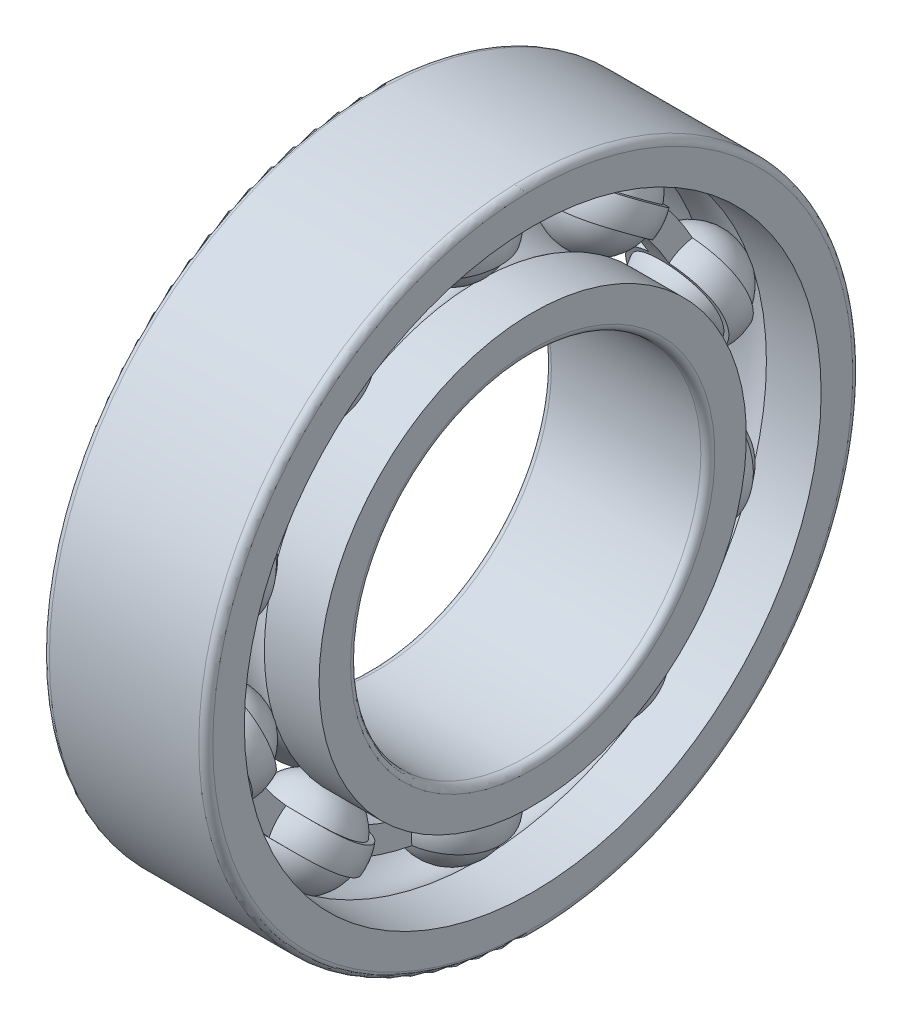
from build123d import *

# Parameters (mm, degrees)
SKETCH_2_W               = 0.87318
SKETCH_2_H               = 1.091475
PATTERN_CIRCULAR_1_COUNT = 10
SKETCH_4_W               = 4.3659
SKETCH_4_H               = 2.18295
SKETCH_5_W               = 4.3659
SKETCH_5_H               = 2.18295
PATTERN_CIRCULAR_2_COUNT = 10


with BuildPart() as part:
    # 草图2 → Revolve 262 (revolve)
    with BuildSketch(Plane.XY, mode=Mode.PRIVATE) as revolve_262_sk:
        with Locations((0, 10.75)):
            Rectangle(SKETCH_2_W, SKETCH_2_H)
    revolve(revolve_262_sk.sketch.rotate(Axis((-12.420610377, 0, 0), (1, 0, 0)), 90), axis=Axis((-12.420610377, 0, 0), (1, 0, 0)))

    # 草图3 → 凸台-旋转1 (revolve)
    with BuildSketch(Plane.XY):
        with BuildLine():
            Line((-2.18295, 10.75), (2.18295, 10.75))
            ThreePointArc((2.18295, 10.75), (0, 8.56705), (-2.18295, 10.75))
        make_face()
    revolve_1 = revolve(axis=Axis((-5.568093779, 10.75, 0), (1, 0, 0)))

    # 阵列(圆周)1: 凸台-旋转1 ×10 about axis
    pattern_circular_1_axis = Axis((0, 0, 0), (1, 0, 0))
    for i in range(1, PATTERN_CIRCULAR_1_COUNT):
        add(revolve_1.rotate(pattern_circular_1_axis, i * 360 / PATTERN_CIRCULAR_1_COUNT))

    # 草图4 → 切除-旋转1 (revolve, cut)
    with BuildSketch(Plane.XY, mode=Mode.PRIVATE) as cut_revolve_1_sk:
        with Locations((0, 12.3872125)):
            Rectangle(SKETCH_4_W, SKETCH_4_H)
    revolve(cut_revolve_1_sk.sketch.rotate(Axis((0, 0, 0), (1, 0, 0)), 82.768656666), axis=Axis((0, 0, 0), (1, 0, 0)), mode=Mode.SUBTRACT)

    # 草图5 → 切除-旋转2 (revolve, cut)
    with BuildSketch(Plane.XY, mode=Mode.PRIVATE) as cut_revolve_2_sk:
        with Locations((0, 9.1127875)):
            Rectangle(SKETCH_5_W, SKETCH_5_H)
    revolve(cut_revolve_2_sk.sketch.rotate(Axis((0, 0, 0), (1, 0, 0)), 96.668258617), axis=Axis((0, 0, 0), (1, 0, 0)), mode=Mode.SUBTRACT)

    # 草图6 → 凸台-旋转2 (revolve)
    with BuildSketch(Plane.XY):
        with BuildLine():
            Line((-1.9845, 10.75), (1.9845, 10.75))
            ThreePointArc((1.9845, 10.75), (0, 8.7655), (-1.9845, 10.75))
        make_face()
    revolve_2 = revolve(axis=Axis((-5.568093779, 10.75, 0), (1, 0, 0)))

    # 阵列(圆周)2: 凸台-旋转2 ×10 about axis
    pattern_circular_2_axis = Axis((0, 0, 0), (1, 0, 0))
    for i in range(1, PATTERN_CIRCULAR_2_COUNT):
        add(revolve_2.rotate(pattern_circular_2_axis, i * 360 / PATTERN_CIRCULAR_2_COUNT))

    # 草图7 → 凸台-旋转3 (revolve)
    with BuildSketch(Plane.XY, mode=Mode.PRIVATE) as revolve_3_sk:
        with BuildLine():
            Line((-3.2, 14), (3.2, 14))
            ThreePointArc((3.2, 14), (3.412132034, 13.912132034), (3.5, 13.7))
            Line((3.5, 13.7), (3.5, 12.35))
            Line((3.5, 12.35), (1.15700054, 12.35))
            ThreePointArc((1.15700054, 12.35), (0, 12.7245), (-1.15700054, 12.35))
            Line((-1.15700054, 12.35), (-3.5, 12.35))
            Line((-3.5, 12.35), (-3.5, 13.7))
            ThreePointArc((-3.5, 13.7), (-3.412132034, 13.912132034), (-3.2, 14))
        make_face()
    revolve(revolve_3_sk.sketch.rotate(Axis((0, 0, 0), (1, 0, 0)), 90), axis=Axis((0, 0, 0), (1, 0, 0)))

    # 草图8 → 凸台-旋转4 (revolve)
    with BuildSketch(Plane.XY, mode=Mode.PRIVATE) as revolve_4_sk:
        with BuildLine():
            Line((-3.5, 9.15), (-1.15700054, 9.15))
            ThreePointArc((-1.15700054, 9.15), (0, 8.7755), (1.15700054, 9.15))
            Line((1.15700054, 9.15), (3.5, 9.15))
            Line((3.5, 9.15), (3.5, 7.8))
            ThreePointArc((3.5, 7.8), (3.412132034, 7.587867966), (3.2, 7.5))
            Line((3.2, 7.5), (-3.2, 7.5))
            ThreePointArc((-3.2, 7.5), (-3.412132034, 7.587867966), (-3.5, 7.8))
            Line((-3.5, 7.8), (-3.5, 9.15))
        make_face()
    revolve(revolve_4_sk.sketch.rotate(Axis((-12.420610377, 0, 0), (1, 0, 0)), 90), axis=Axis((-12.420610377, 0, 0), (1, 0, 0)))


solid = part.part
